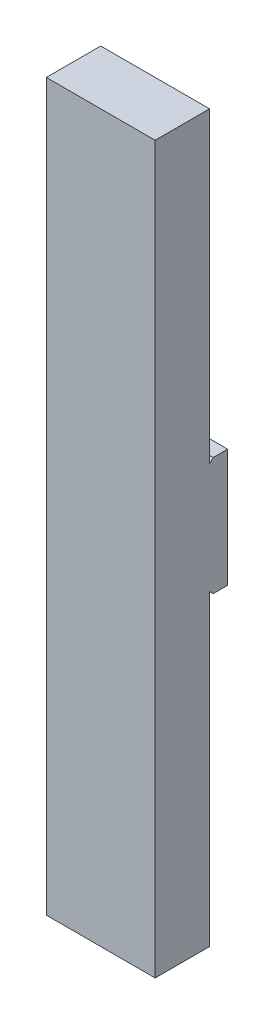
SolidWorks part; units mm, degrees
ref_plane "前视基准面" through (0, 0, 0) normal (0, 0, 1) x (1, 0, 0)
ref_plane "上视基准面" through (0, 0, 0) normal (0, 1, 0) x (1, 0, 0)
ref_plane "右视基准面" through (0, 0, 0) normal (1, 0, 0) x (0, 0, -1)
sketch "草图1" plane through (0, 0, 0) normal (0, 0, 1) x (1, 0, 0)
  line L1 (-60, 32.5) -> (60, 32.5)
  line L2 (-60, 32.5) -> (-60, -32.5)
  line L3 (-60, -32.5) -> (60, -32.5)
  line L4 (60, 32.5) -> (60, -32.5)
  line L5 (-60, 32.5) -> (60, -32.5) construction
  line L6 (-60, -32.5) -> (60, 32.5) construction
  point P0 (0, 0)
  dimension "D1" = 120
  dimension "D2" = 65
extrude "凸台-拉伸1" add sketch "草图1" along normal blind 10
chamfer "倒角1" distance 2 angle 45 4 edges at (60, 0, 10) (0, -32.5, 10) (-60, 0, 10) (0, 32.5, 10)
sketch "草图2" plane through (0, 0, 10) normal (0, 0, 1) x (1, 0, 0)
  line L1 (-60, 32.5) -> (60, 32.5)
  line L2 (-60, 32.5) -> (-60, -32.5)
  line L3 (-60, -32.5) -> (60, -32.5)
  line L4 (60, 32.5) -> (60, -32.5)
  line L5 (-60, 32.5) -> (60, -32.5) construction
  line L6 (-60, -32.5) -> (60, 32.5) construction
  point P0 (0, 0)
extrude "凸台-拉伸2" add sketch "草图2" along normal blind 30
sketch "草图3" plane through (0, 0, 0) normal (0, 0, -1) x (-1, 0, 0)
  circle A0 centre (-32.5, 0) radius 10
  dimension "D1" = 20
extrude "切除-拉伸1" cut sketch "草图3" against normal blind 2
hole_wizard "M6 六角头螺栓的柱形沉头孔1" positions "草图4" profile "草图5" counterbore size "M6" standard "GB" end condition through all
sketch "草图4" plane through (0, 0, 40) normal (0, 0, 1) x (1, 0, 0)
  point P0 (32.5, 0)
sketch "草图5" plane through (32.5, 0, 40) normal (1, 0, 0) x (0, -1, 0)
  line L0 (0, 0) -> (0, 40)
  line L1 (0, 40) -> (3.3, 40)
  line L3 (3.3, 40) -> (3.3, 35)
  line L4 (3.3, 35) -> (6.5, 35)
  line L5 (6.5, 35) -> (6.5, 0)
  line L7 (6.5, 0) -> (0, 0)
  line L11 (0, -6.35) -> (0, 107.95) construction
  dimension "通孔孔直径" = 6.6
  dimension "通孔孔深度" = 40
  dimension "柱形沉头孔直径" = 13
  dimension "柱形沉头孔深度" = 35
sketch "草图6" plane through (0, 0, 40) normal (0, 0, 1) x (1, 0, 0)
  line L0 (-60, 32.5) -> (-60, -32.5) construction
  line L1 (0, 200) -> (-60, 200)
  line L2 (0, 200) -> (0, -200)
  line L3 (0, -200) -> (-60, -200)
  line L4 (-60, 200) -> (-60, -200)
  line L5 (0, 200) -> (-60, -200) construction
  line L6 (0, -200) -> (-60, 200) construction
  point P0 (-30, 0)
  point P7 (0, 0)
  dimension "D1" = 60
  dimension "D2" = 30
  dimension "D3" = 400
extrude "凸台-拉伸3" add sketch "草图6" against normal up to surface (30 mm away) up to face at (0, 0, 10)
sketch "草图7" plane through (0, 0, 40) normal (0, 0, 1) x (1, 0, 0)
  line L0 (0, 32.5) -> (0, 200) construction
  line L1 (0, 32.5) -> (60, 32.5)
  line L2 (0, 32.5) -> (0, -32.5)
  line L3 (0, -32.5) -> (60, -32.5)
  line L4 (60, 32.5) -> (60, -32.5)
  line L5 (60, -32.5) -> (60, 32.5) construction
  line L6 (0, -32.5) -> (60, -32.5) construction
extrude "切除-拉伸2" cut sketch "草图7" against normal up to surface (40 mm away) up to face at (22.5, 0, 0)
